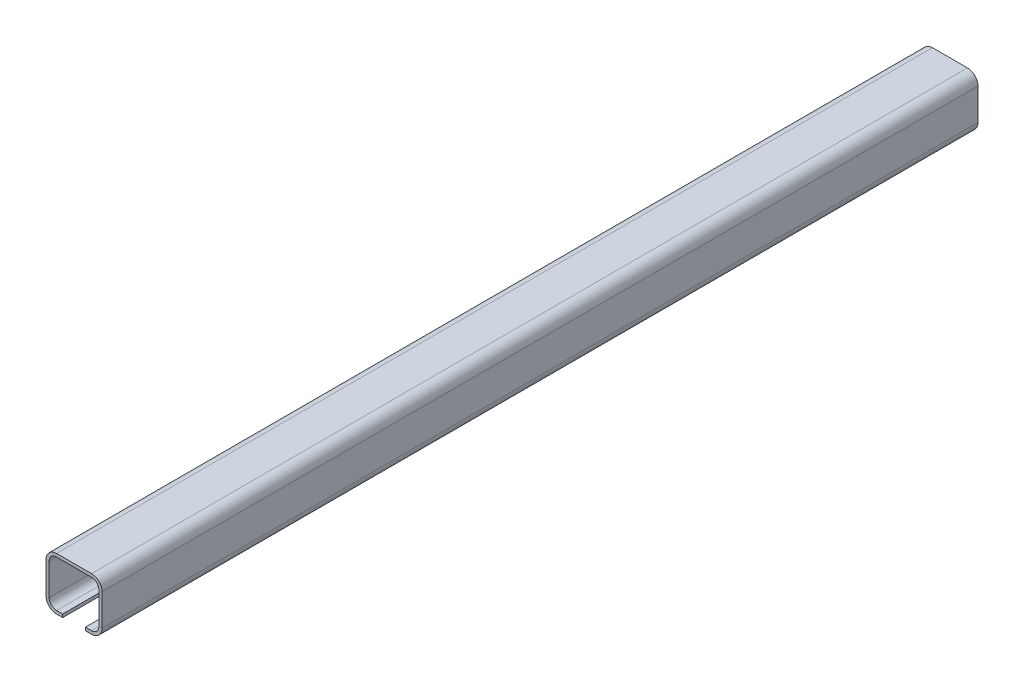
SolidWorks part; units mm, degrees
ref_plane "Front Plane" through (0, 0, 0) normal (0, 0, 1) x (1, 0, 0)
ref_plane "Top Plane" through (0, 0, 0) normal (0, 1, 0) x (1, 0, 0)
ref_plane "Right Plane" through (0, 0, 0) normal (1, 0, 0) x (0, 0, -1)
other "Configuration Table"
sketch "Sketch1" plane through (0, 0, 0) normal (0, 0, 1) x (1, 0, 0)
  line L0 (-10, -13.2) -> (-6.5, -13.2)
  line L1 (-10, 15) -> (10, 15)
  line L2 (-16, 9) -> (-16, -9)
  line L3 (-10, -15) -> (-6.5, -15)
  line L4 (16, 9) -> (16, -9)
  line L5 (-16, 15) -> (16, -15) construction
  line L6 (-16, -15) -> (16, 15) construction
  line L7 (-14.2, 9) -> (-14.2, -9)
  line L8 (6.5, -15) -> (10, -15)
  line L9 (-10, 13.2) -> (10, 13.2)
  line L10 (14.2, 9) -> (14.2, -9)
  line L11 (6.5, -13.2) -> (10, -13.2)
  line L12 (-6.5, -15) -> (-6.5, -13.2)
  line L13 (6.5, -15) -> (6.5, -13.2)
  arc A0 (-16, -9) -> (-10, -15) centre (-10, -9) ccw
  arc A1 (10, -15) -> (16, -9) centre (10, -9) ccw
  arc A2 (10, 15) -> (16, 9) centre (10, 9) cw
  arc A3 (-10, 15) -> (-16, 9) centre (-10, 9) ccw
  arc A4 (-14.2, -9) -> (-10, -13.2) centre (-10, -9) ccw
  arc A5 (-10, 13.2) -> (-14.2, 9) centre (-10, 9) ccw
  arc A6 (10, 13.2) -> (14.2, 9) centre (10, 9) cw
  arc A7 (10, -13.2) -> (14.2, -9) centre (10, -9) ccw
  point P0 (0, 0)
  dimension "D5" = 6
  dimension "D1" = 32
  dimension "D2" = 30
  dimension "D3" = 9.5
  dimension "D4" = 9.5
  dimension "D6" = 1.8
extrude "Boss-Extrude1" add sketch "Sketch1" along normal blind 500
